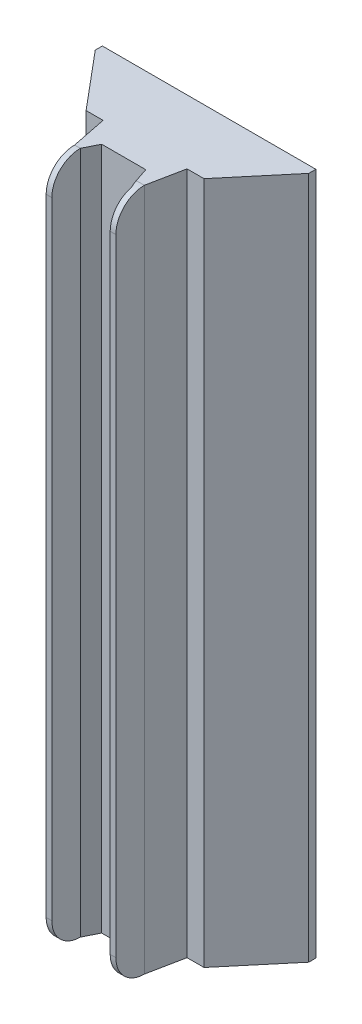
from build123d import *

# Parameters (mm, degrees)
BOSS_EXTRUDE1_DEPTH = 48
CHAMFER1_SIZE       = 1
CHAMFER1_SIZE2      = 0.5
CHAMFER2_SIZE       = 0.5
CHAMFER2_SIZE2      = 1.5
CHAMFER3_SIZE       = 0.5
CHAMFER3_SIZE2      = 2.5
CHAMFER4_SIZE       = 2.5
CHAMFER4_SIZE2      = 0.5
CHAMFER5_SIZE       = 4
CHAMFER5_SIZE2      = 3.356398525
CHAMFER6_SIZE       = 4
CHAMFER6_SIZE2      = 3.356398525
FILLET1_R           = 2


with BuildPart() as part:
    # Sketch1 → Boss-Extrude1 (new body)
    with BuildSketch(Plane(origin=(0, 0, 0), x_dir=(1, 0, 0), z_dir=(0, 1, 0))):
        Polygon((-7.5, 2.25), (7.5, 2.25), (7.5, -2.25), (2.45, -2.25), (2.45, -6.75), (2.05, -6.75), (2.05, -3.75), (-2.05, -3.75), (-2.05, -6.75), (-2.45, -6.75), (-2.45, -2.25), (-7.5, -2.25), align=None)
    extrude(amount=BOSS_EXTRUDE1_DEPTH)

    # Chamfer1
    chamfer1_edges = [part.edges().sort_by_distance(p)[0] for p in [
        (-2.05, 24, 3.75),
    ]]
    chamfer1_side = [part.faces().sort_by_distance(p)[0] for p in [
        (-2.05, 24, 5.25),
    ]]
    chamfer(chamfer1_edges, length=CHAMFER1_SIZE, length2=CHAMFER1_SIZE2, reference=chamfer1_side[0])

    # Chamfer2
    chamfer2_edges = [part.edges().sort_by_distance(p)[0] for p in [
        (2.05, 24, 3.75),
    ]]
    chamfer2_side = [part.faces().sort_by_distance(p)[0] for p in [
        (0.25, 24, 3.75),
    ]]
    chamfer(chamfer2_edges, length=CHAMFER2_SIZE, length2=CHAMFER2_SIZE2, reference=chamfer2_side[0])

    # Chamfer3
    chamfer3_edges = [part.edges().sort_by_distance(p)[0] for p in [
        (-2.45, 24, 2.25),
    ]]
    chamfer3_side = [part.faces().sort_by_distance(p)[0] for p in [
        (-4.975, 24, 2.25),
    ]]
    chamfer(chamfer3_edges, length=CHAMFER3_SIZE, length2=CHAMFER3_SIZE2, reference=chamfer3_side[0])

    # Chamfer4
    chamfer4_edges = [part.edges().sort_by_distance(p)[0] for p in [
        (2.45, 24, 2.25),
    ]]
    chamfer4_side = [part.faces().sort_by_distance(p)[0] for p in [
        (2.45, 24, 4.5),
    ]]
    chamfer(chamfer4_edges, length=CHAMFER4_SIZE, length2=CHAMFER4_SIZE2, reference=chamfer4_side[0])

    # Chamfer5
    chamfer5_edges = [part.edges().sort_by_distance(p)[0] for p in [
        (-7.5, 24, 2.25),
    ]]
    chamfer5_side = [part.faces().sort_by_distance(p)[0] for p in [
        (-7.5, 24, 0),
    ]]
    chamfer(chamfer5_edges, length=CHAMFER5_SIZE, length2=CHAMFER5_SIZE2, reference=chamfer5_side[0])

    # Chamfer6
    chamfer6_edges = [part.edges().sort_by_distance(p)[0] for p in [
        (7.5, 24, 2.25),
    ]]
    chamfer6_side = [part.faces().sort_by_distance(p)[0] for p in [
        (7.5, 24, 0),
    ]]
    chamfer(chamfer6_edges, length=CHAMFER6_SIZE, length2=CHAMFER6_SIZE2, reference=chamfer6_side[0])

    # Fillet1
    fillet1_edges = [part.edges().sort_by_distance(p)[0] for p in [
        (-2.25, 0, 6.75),
        (2.25, 0, 6.75),
        (-2.25, 48, 6.75),
        (2.25, 48, 6.75),
    ]]
    fillet(fillet1_edges, radius=FILLET1_R)


solid = part.part
